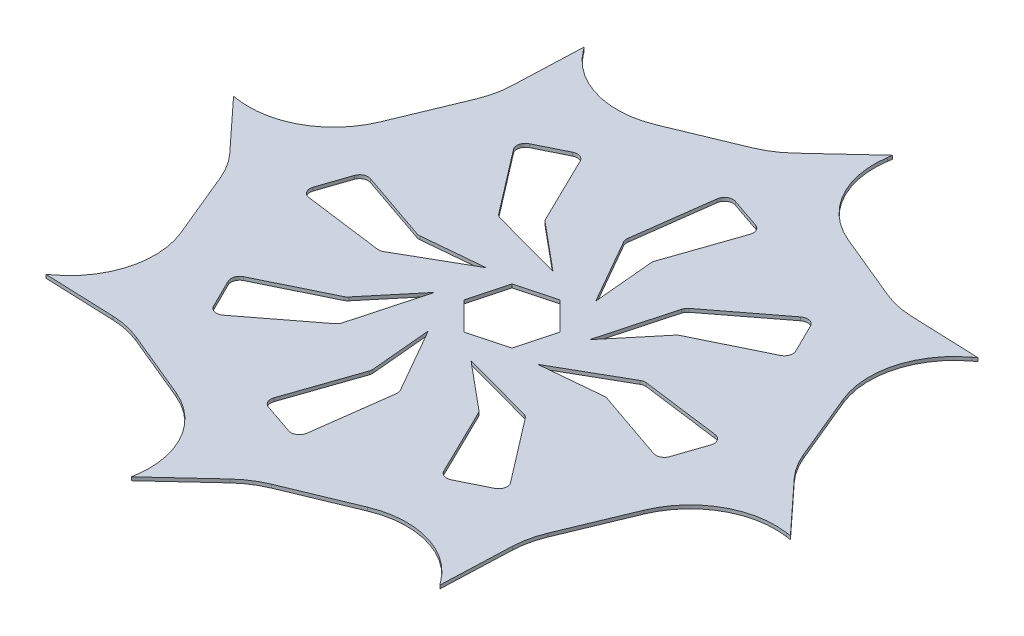
SolidWorks part; units mm, degrees
material "45"
ref_plane "Front Plane" through (0, 0, 0) normal (0, 0, 1) x (1, 0, 0)
ref_plane "Top Plane" through (0, 0, 0) normal (0, 1, 0) x (1, 0, 0)
ref_plane "Right Plane" through (0, 0, 0) normal (1, 0, 0) x (0, 0, -1)
sketch "Sketch1" plane through (0, 0, 0) normal (0, 1, 0) x (1, 0, 0)
  line L1 (114.805, -114.805) -> (162.3588, 0)
  line L2 (162.3588, 0) -> (114.805, 114.805)
  line L3 (114.805, 114.805) -> (0, 162.3588)
  line L4 (0, 162.3588) -> (-114.805, 114.805)
  line L5 (-114.805, 114.805) -> (-162.3588, 0)
  line L6 (-162.3588, 0) -> (-114.805, -114.805)
  line L7 (-114.805, -114.805) -> (0, -162.3588)
  line L8 (0, -162.3588) -> (114.805, -114.805)
  circle A0 centre (0, 0) radius 150 construction
  dimension "D1" = 300
extrude "Boss-Extrude1" add sketch "Sketch1" along normal blind 2
sketch "Sketch2" plane through (0, 2, 0) normal (0, 1, 0) x (1, 0, 0)
  line L0 (0, 0) -> (59.4225, 0) construction
  line L1 (5.9772, 22.3071) -> (-16.3299, 16.3299)
  line L2 (-16.3299, 16.3299) -> (-22.3071, -5.9772)
  line L3 (-22.3071, -5.9772) -> (-5.9772, -22.3071)
  line L4 (-5.9772, -22.3071) -> (16.3299, -16.3299)
  line L5 (16.3299, -16.3299) -> (22.3071, 5.9772)
  line L6 (22.3071, 5.9772) -> (5.9772, 22.3071)
  line L7 (0, 0) -> (22.3071, 5.9772) construction
  circle A0 centre (0, 0) radius 20 construction
  dimension "D1" = 40
  dimension "D2" = 15
extrude "Cut-Extrude1" cut sketch "Sketch2" against normal blind 10
sketch "Sketch3" plane through (0, 2, 0) normal (0, 1, 0) x (1, 0, 0)
  line L0 (7.1807, 123.975) -> (25.2073, 117.8588)
  line L1 (28.3287, 111.4971) -> (13.9987, 69.8505)
  line L2 (13.7476, 67.7664) -> (17.0204, 32.1308)
  line L3 (17.0204, 32.1308) -> (-4.8848, 70.4296)
  line L4 (-5.5015, 73.5667) -> (0.6173, 119.8948)
  line L5 (92.7411, 82.586) -> (101.163, 65.5145)
  line L6 (98.8718, 58.8089) -> (59.2903, 39.4932)
  line L7 (57.6391, 38.197) -> (34.7552, 10.6847)
  line L8 (34.7552, 10.6847) -> (46.3472, 53.2553)
  line L9 (48.1294, 55.9097) -> (85.2149, 84.3419)
  line L10 (123.975, -7.1807) -> (117.8588, -25.2073)
  line L11 (111.4971, -28.3287) -> (69.8505, -13.9987)
  line L12 (67.7664, -13.7476) -> (32.1308, -17.0204)
  line L13 (32.1308, -17.0204) -> (70.4296, 4.8848)
  line L14 (73.5667, 5.5015) -> (119.8948, -0.6173)
  line L15 (82.586, -92.7411) -> (65.5145, -101.163)
  line L16 (58.8089, -98.8718) -> (39.4932, -59.2903)
  line L17 (38.197, -57.6391) -> (10.6847, -34.7552)
  line L18 (10.6847, -34.7552) -> (53.2553, -46.3472)
  line L19 (55.9097, -48.1294) -> (84.3419, -85.2149)
  line L20 (-7.1807, -123.975) -> (-25.2073, -117.8588)
  line L21 (-28.3287, -111.4971) -> (-13.9987, -69.8505)
  line L22 (-13.7476, -67.7664) -> (-17.0204, -32.1308)
  line L23 (-17.0204, -32.1308) -> (4.8848, -70.4296)
  line L24 (5.5015, -73.5667) -> (-0.6173, -119.8948)
  line L25 (-92.7411, -82.586) -> (-101.163, -65.5145)
  line L26 (-98.8718, -58.8089) -> (-59.2903, -39.4932)
  line L27 (-57.6391, -38.197) -> (-34.7552, -10.6847)
  line L28 (-34.7552, -10.6847) -> (-46.3472, -53.2553)
  line L29 (-48.1294, -55.9097) -> (-85.2149, -84.3419)
  line L30 (-123.975, 7.1807) -> (-117.8588, 25.2073)
  line L31 (-111.4971, 28.3287) -> (-69.8505, 13.9987)
  line L32 (-67.7664, 13.7476) -> (-32.1308, 17.0204)
  line L33 (-32.1308, 17.0204) -> (-70.4296, -4.8848)
  line L34 (-73.5667, -5.5015) -> (-119.8948, 0.6173)
  line L35 (-82.586, 92.7411) -> (-65.5145, 101.163)
  line L36 (-58.8089, 98.8718) -> (-39.4932, 59.2903)
  line L37 (-38.197, 57.6391) -> (-10.6847, 34.7552)
  line L38 (-10.6847, 34.7552) -> (-53.2553, 46.3472)
  line L39 (-55.9097, 48.1294) -> (-84.3419, 85.2149)
  arc A0 (13.9987, 69.8505) -> (13.7476, 67.7664) centre (18.7267, 68.2237) ccw
  arc A1 (-4.8848, 70.4296) -> (-5.5015, 73.5667) centre (-0.5445, 72.912) cw
  arc A2 (0.6173, 119.8948) -> (7.1807, 123.975) centre (5.5743, 119.2401) cw
  arc A3 (28.3287, 111.4971) -> (25.2073, 117.8588) centre (23.6008, 113.1239) ccw
  circle A4 centre (0, 0) radius 14.7187 construction
  arc A5 (59.2903, 39.4932) -> (57.6391, 38.197) centre (61.4832, 34.9997) ccw
  arc A6 (46.3472, 53.2553) -> (48.1294, 55.9097) centre (51.1715, 51.9416) cw
  arc A7 (85.2149, 84.3419) -> (92.7411, 82.586) centre (88.2571, 80.3739) cw
  arc A8 (98.8718, 58.8089) -> (101.163, 65.5145) centre (96.679, 63.3024) ccw
  arc A9 (69.8505, -13.9987) -> (67.7664, -13.7476) centre (68.2237, -18.7267) ccw
  arc A10 (70.4296, 4.8848) -> (73.5667, 5.5015) centre (72.912, 0.5445) cw
  arc A11 (119.8948, -0.6173) -> (123.975, -7.1807) centre (119.2401, -5.5743) cw
  arc A12 (111.4971, -28.3287) -> (117.8588, -25.2073) centre (113.1239, -23.6008) ccw
  arc A13 (39.4932, -59.2903) -> (38.197, -57.6391) centre (34.9997, -61.4832) ccw
  arc A14 (53.2553, -46.3472) -> (55.9097, -48.1294) centre (51.9416, -51.1715) cw
  arc A15 (84.3419, -85.2149) -> (82.586, -92.7411) centre (80.3739, -88.2571) cw
  arc A16 (58.8089, -98.8718) -> (65.5145, -101.163) centre (63.3024, -96.679) ccw
  arc A17 (-13.9987, -69.8505) -> (-13.7476, -67.7664) centre (-18.7267, -68.2237) ccw
  arc A18 (4.8848, -70.4296) -> (5.5015, -73.5667) centre (0.5445, -72.912) cw
  arc A19 (-0.6173, -119.8948) -> (-7.1807, -123.975) centre (-5.5743, -119.2401) cw
  arc A20 (-28.3287, -111.4971) -> (-25.2073, -117.8588) centre (-23.6008, -113.1239) ccw
  arc A21 (-59.2903, -39.4932) -> (-57.6391, -38.197) centre (-61.4832, -34.9997) ccw
  arc A22 (-46.3472, -53.2553) -> (-48.1294, -55.9097) centre (-51.1715, -51.9416) cw
  arc A23 (-85.2149, -84.3419) -> (-92.7411, -82.586) centre (-88.2571, -80.3739) cw
  arc A24 (-98.8718, -58.8089) -> (-101.163, -65.5145) centre (-96.679, -63.3024) ccw
  arc A25 (-69.8505, 13.9987) -> (-67.7664, 13.7476) centre (-68.2237, 18.7267) ccw
  arc A26 (-70.4296, -4.8848) -> (-73.5667, -5.5015) centre (-72.912, -0.5445) cw
  arc A27 (-119.8948, 0.6173) -> (-123.975, 7.1807) centre (-119.2401, 5.5743) cw
  arc A28 (-111.4971, 28.3287) -> (-117.8588, 25.2073) centre (-113.1239, 23.6008) ccw
  arc A29 (-39.4932, 59.2903) -> (-38.197, 57.6391) centre (-34.9997, 61.4832) ccw
  arc A30 (-53.2553, 46.3472) -> (-55.9097, 48.1294) centre (-51.9416, 51.1715) cw
  arc A31 (-84.3419, 85.2149) -> (-82.586, 92.7411) centre (-80.3739, 88.2571) cw
  arc A32 (-58.8089, 98.8718) -> (-65.5145, 101.163) centre (-63.3024, 96.679) ccw
  point P110 (0, 0)
  dimension "D1" = 5
  dimension "D2" = 8
extrude "Cut-Extrude2" cut sketch "Sketch3" against normal blind 10
sketch "Sketch6" plane through (0, 2, 0) normal (0, 1, 0) x (1, 0, 0)
  line L0 (0, 0) -> (-114.805, 114.805) construction
  line L1 (-117.5739, 108.1204) -> (-115.6573, 158.0837)
  line L2 (-114.805, 114.805) -> (-162.3588, 0) construction
  line L3 (-115.6573, 158.0837) -> (-90.8359, 124.7334)
  line L4 (0, 162.3588) -> (-114.805, 114.805) construction
  line L5 (-90.8359, 124.7334) -> (-114.805, 114.805)
  line L6 (-114.805, 114.805) -> (-117.5739, 108.1204)
  line L7 (-6.6846, 159.59) -> (30, 193.5641)
  line L8 (30, 193.5641) -> (23.9692, 152.4305)
  line L9 (23.9692, 152.4305) -> (0, 162.3588)
  line L10 (0, 162.3588) -> (-6.6846, 159.59)
  line L11 (0, 0) -> (0, 162.3588) construction
  line L12 (108.1204, 117.5739) -> (158.0837, 115.6573)
  line L13 (158.0837, 115.6573) -> (124.7334, 90.8359)
  line L14 (124.7334, 90.8359) -> (114.805, 114.805)
  line L15 (114.805, 114.805) -> (108.1204, 117.5739)
  line L16 (0, 0) -> (114.805, 114.805) construction
  line L17 (159.59, 6.6846) -> (193.5641, -30)
  line L18 (193.5641, -30) -> (152.4305, -23.9692)
  line L19 (152.4305, -23.9692) -> (162.3588, 0)
  line L20 (162.3588, 0) -> (159.59, 6.6846)
  line L21 (0, 0) -> (162.3588, 0) construction
  line L22 (117.5739, -108.1204) -> (115.6573, -158.0837)
  line L23 (115.6573, -158.0837) -> (90.8359, -124.7334)
  line L24 (90.8359, -124.7334) -> (114.805, -114.805)
  line L25 (114.805, -114.805) -> (117.5739, -108.1204)
  line L26 (0, 0) -> (114.805, -114.805) construction
  line L27 (6.6846, -159.59) -> (-30, -193.5641)
  line L28 (-30, -193.5641) -> (-23.9692, -152.4305)
  line L29 (-23.9692, -152.4305) -> (0, -162.3588)
  line L30 (0, -162.3588) -> (6.6846, -159.59)
  line L31 (0, 0) -> (0, -162.3588) construction
  line L32 (-108.1204, -117.5739) -> (-158.0837, -115.6573)
  line L33 (-158.0837, -115.6573) -> (-124.7334, -90.8359)
  line L34 (-124.7334, -90.8359) -> (-114.805, -114.805)
  line L35 (-114.805, -114.805) -> (-108.1204, -117.5739)
  line L36 (0, 0) -> (-114.805, -114.805) construction
  line L37 (-159.59, -6.6846) -> (-193.5641, 30)
  line L38 (-193.5641, 30) -> (-152.4305, 23.9692)
  line L39 (-152.4305, 23.9692) -> (-162.3588, 0)
  line L40 (-162.3588, 0) -> (-159.59, -6.6846)
  line L41 (0, 0) -> (-162.3588, 0) construction
  circle A0 centre (0, 0) radius 96.6837 construction
  point P27 (0, 0)
  dimension "D1" = 8
  dimension "D2" = 50
  dimension "D3" = 30
extrude "Boss-Extrude2" add sketch "Sketch6" against normal blind 2
fillet "Fillet1" radius 50 16 edges at (-117.5739, 1, -108.1204) (-90.8359, 1, -124.7334) (-6.6846, 1, -159.59) (23.9692, 1, -152.4305) (108.1204, 1, -117.5739) (124.7334, 1, -90.8359) (159.59, 1, -6.6846) (152.4305, 1, 23.9692) (117.5739, 1, 108.1204) (90.8359, 1, 124.7334) (6.6846, 1, 159.59) (-23.9692, 1, 152.4305) (-108.1204, 1, 117.5739) (-124.7334, 1, 90.8359) (-159.59, 1, 6.6846) (-152.4305, 1, -23.9692)
